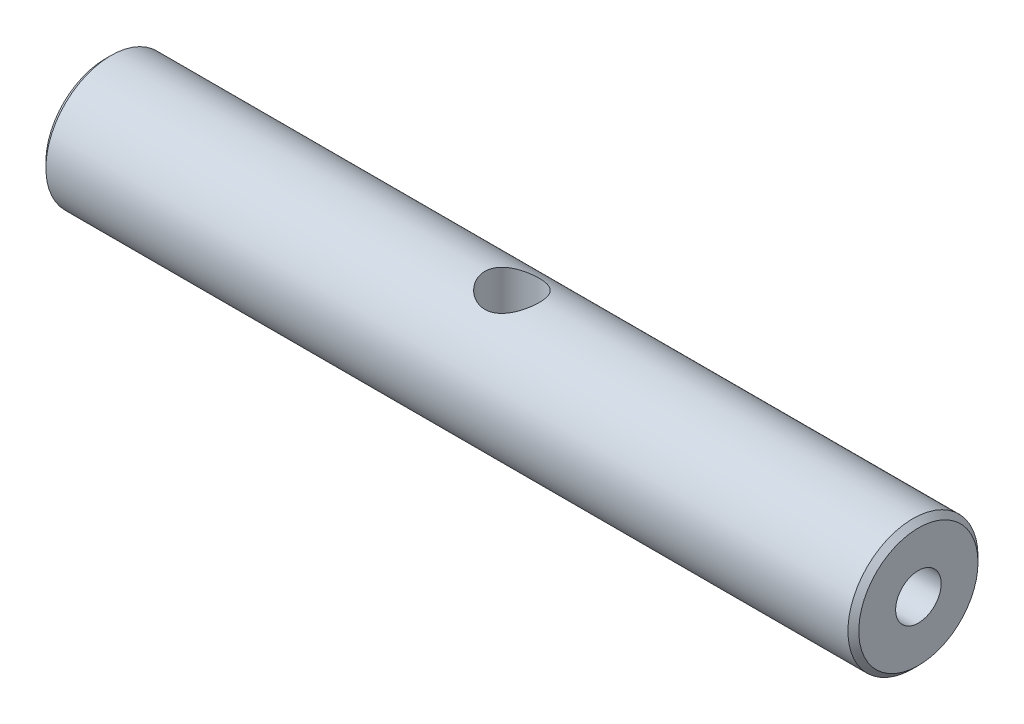
SolidWorks part; units mm, degrees
ref_plane "Front" through (0, 0, 0) normal (0, 0, 1) x (1, 0, 0)
ref_plane "Top" through (0, 0, 0) normal (0, 1, 0) x (1, 0, 0)
ref_plane "Right" through (0, 0, 0) normal (1, 0, 0) x (0, 0, -1)
sketch "Sketch1" plane through (0, 0, 0) normal (1, 0, 0) x (0, 0, -1)
  circle A0 centre (0, 0) radius 6
  dimension "D1" = 12
extrude "Boss-Extrude1" add sketch "Sketch1" along normal blind 75
hole_wizard "M5 Tapped Hole1" positions "Sketch3" profile "Sketch2" tap size "M5" standard "GB"
sketch "Sketch3" plane through (75, 0, 0) normal (1, 0, 0) x (0, 0, -1)
  point P0 (0, 0)
sketch "Sketch2" plane through (75, 0, 0) normal (0, 1, 0) x (0, 0, -1)
  line L0 (0, 0) -> (0, 13.6618)
  line L1 (0, 13.6618) -> (2.1, 12.4)
  line L2 (2.1, 12.4) -> (2.1, 0)
  line L5 (2.1, 0) -> (0, 0)
  line L10 (0, 13.6618) -> (-2.1, 12.4) construction
  line L11 (0, -6.35) -> (0, 107.95) construction
  dimension "螺纹孔钻头直径" = 4.2
  dimension "螺纹孔钻头深度" = 12.4
  dimension "导头角度" = 118
cosmetic thread "Cosmetic Thread1" parameters "D1"=10, "D2"=5
hole_wizard "M5 Tapped Hole2" positions "Sketch5" profile "Sketch4" tap size "M5" standard "GB"
sketch "Sketch5" plane through (0, 0, 0) normal (-1, 0, 0) x (0, 0, 1)
  point P0 (0, 0)
sketch "Sketch4" plane through (0, 0, 0) normal (0, 1, 0) x (0, 0, 1)
  line L0 (0, 0) -> (0, 13.6618)
  line L1 (0, 13.6618) -> (2.1, 12.4)
  line L2 (2.1, 12.4) -> (2.1, 0)
  line L5 (2.1, 0) -> (0, 0)
  line L10 (0, 13.6618) -> (-2.1, 12.4) construction
  line L11 (0, -6.35) -> (0, 107.95) construction
  dimension "螺纹孔钻头直径" = 4.2
  dimension "螺纹孔钻头深度" = 12.4
  dimension "导头角度" = 118
cosmetic thread "Cosmetic Thread2" parameters "D1"=10, "D2"=5
chamfer "Chamfer1" distance 0.5 angle 45 2 edges at (75, 0, -6) (0, 0, -6)
sketch "Sketch6" plane through (0, 0, 0) normal (0, 1, 0) x (1, 0, 0)
  line L0 (0, 0) -> (75, 0) construction
  line L1 (75, -5.5) -> (75, 5.5) construction
  circle A0 centre (37.5, 0) radius 2.5
  dimension "D1" = 5
extrude "Cut-Extrude1" cut sketch "Sketch6" against normal mid plane 34
